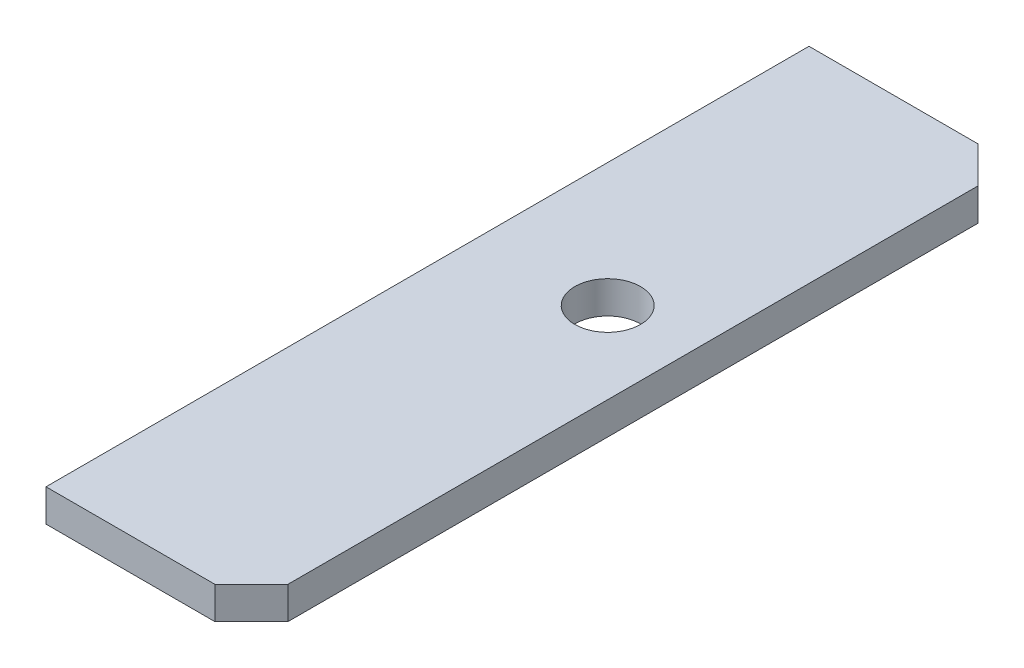
from build123d import *

# Parameters (mm, degrees)
SKETCH3_R           = 14.224
BOSS_EXTRUDE1_DEPTH = 7


with BuildPart() as part:
    # Sketch3 → Boss-Extrude1 (new, symmetric)
    with BuildSketch(Plane(origin=(0, 0, 0), x_dir=(1, 0, 0), z_dir=(0, 1, 0))):
        Polygon((19.556, 140.716), (35.306, 124.966), (35.306, -173.734), (19.556, -189.484), (-53.594, -189.484), (-53.594, 140.716), align=None)
        with Locations(Location((0, 0, 0), (0, 0, 270))):
            Circle(SKETCH3_R, mode=Mode.SUBTRACT)
    extrude(amount=BOSS_EXTRUDE1_DEPTH, both=True)


solid = part.part
